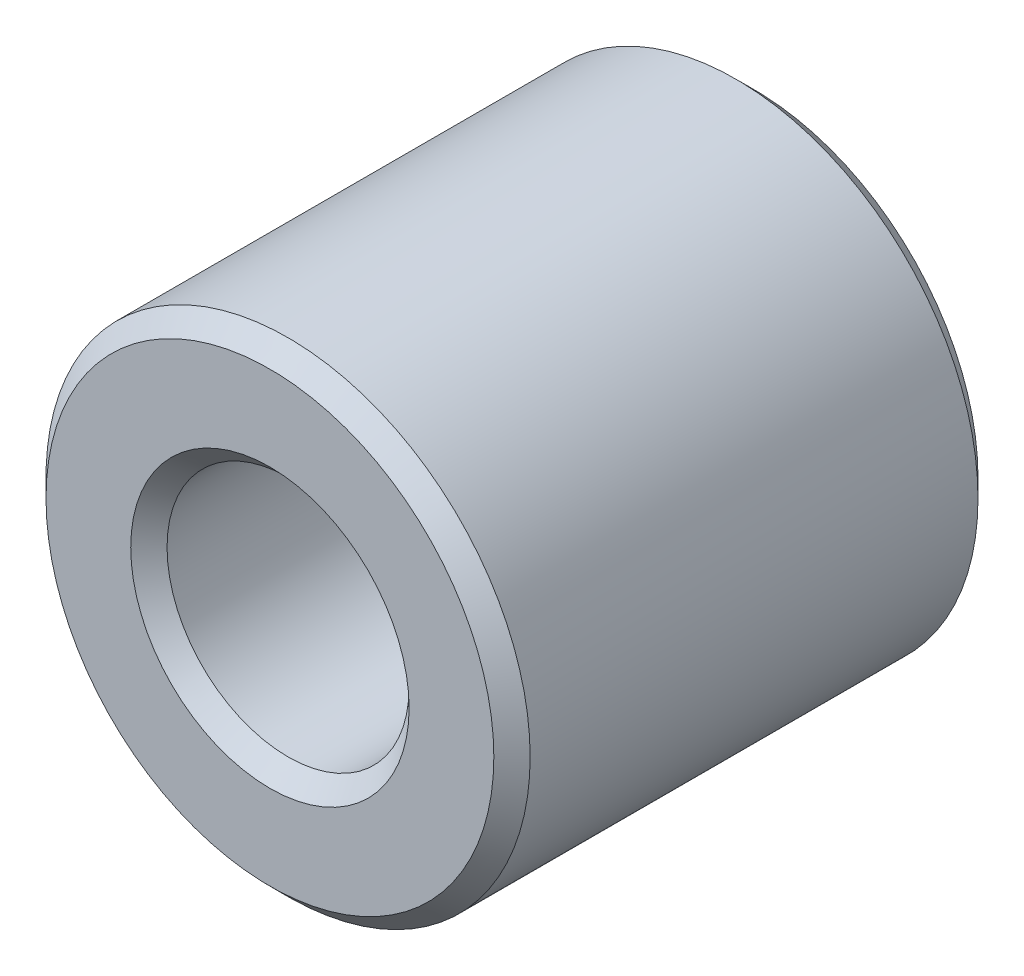
SolidWorks part; units mm, degrees
material "6061 合金"
ref_plane "Front Plane" through (0, 0, 0) normal (0, 0, 1) x (1, 0, 0)
ref_plane "Top Plane" through (0, 0, 0) normal (0, 1, 0) x (1, 0, 0)
ref_plane "Right Plane" through (0, 0, 0) normal (1, 0, 0) x (0, 0, -1)
sketch "Sketch1" plane through (0, 0, 0) normal (0, 0, 1) x (1, 0, 0)
  circle A0 centre (0, 0) radius 4
  circle A1 centre (0, 0) radius 2
  dimension "D1" = 4
  dimension "D2" = 8
extrude "Boss-Extrude1" add sketch "Sketch1" along normal blind 8
chamfer "Chamfer1" distance 0.3 angle 45 4 edges at (2, 0, 0) (2, 0, 8) (4, 0, 0) (4, 0, 8)
